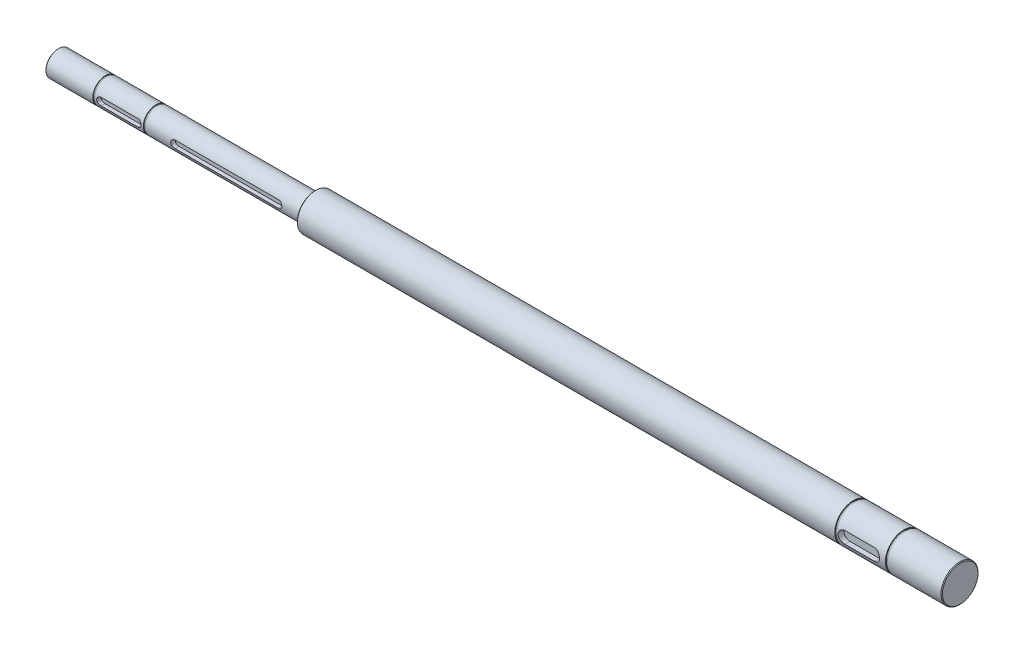
SolidWorks part; units mm, degrees
ref_plane "前视基准面" through (0, 0, 0) normal (0, 0, 1) x (1, 0, 0)
ref_plane "上视基准面" through (0, 0, 0) normal (0, 1, 0) x (1, 0, 0)
ref_plane "右视基准面" through (0, 0, 0) normal (1, 0, 0) x (0, 0, -1)
sketch "草图2" plane through (0, 0, 0) normal (1, 0, 0) x (0, 0, -1)
  circle A0 centre (0, 0) radius 12.5
  dimension "D1" = 25
extrude "凸台-拉伸1" add sketch "草图2" along normal mid plane 609
sketch "草图3" plane through (-304.5, 0, 0) normal (-1, 0, 0) x (0, 0, 1)
  circle A0 centre (0, 0) radius 8.5
  dimension "D1" = 17
extrude "切除-拉伸1" cut sketch "草图3" against normal blind 173.5 flip side to cut
ref_plane "基准面1" through (0, 0, 8.5) normal (0, 0, 1) x (1, 0, 0)
sketch "草图5" plane through (0, 0, 8.5) normal (0, 0, 1) x (1, 0, 0)
  line L0 (-267.5, 0) -> (-242.5, 0) construction
  line L1 (-267.5, 2.5) -> (-242.5, 2.5)
  line L2 (-267.5, -2.5) -> (-242.5, -2.5)
  line L3 (-217.5, 0) -> (-147.5, 0) construction
  line L4 (-217.5, 2.5) -> (-147.5, 2.5)
  line L5 (-217.5, -2.5) -> (-147.5, -2.5)
  line L7 (-304.5, 8.5) -> (-304.5, -8.5) construction
  arc A0 (-267.5, 2.5) -> (-267.5, -2.5) centre (-267.5, 0) ccw
  arc A1 (-242.5, -2.5) -> (-242.5, 2.5) centre (-242.5, 0) ccw
  arc A2 (-217.5, 2.5) -> (-217.5, -2.5) centre (-217.5, 0) ccw
  arc A3 (-147.5, -2.5) -> (-147.5, 2.5) centre (-147.5, 0) ccw
  point P3 (-255, 0)
  point P8 (-182.5, 0)
  dimension "D5" = 25
  dimension "D6" = 49.5
  dimension "D1" = 5
  dimension "D2" = 5
  dimension "D3" = 25
  dimension "D4" = 70
extrude "切除-拉伸2" cut sketch "草图5" against normal blind 3
ref_plane "基准面2" through (0, 0, 12.5) normal (0, 0, 1) x (1, 0, 0)
sketch "草图6" plane through (0, 0, 12.5) normal (0, 0, 1) x (1, 0, 0)
  line L0 (238.5, 0) -> (258.5, 0) construction
  line L1 (238.5, 4) -> (258.5, 4)
  line L2 (238.5, -4) -> (258.5, -4)
  line L3 (304.5, -12.5) -> (304.5, 12.5) construction
  arc A0 (238.5, 4) -> (238.5, -4) centre (238.5, 0) ccw
  arc A1 (258.5, -4) -> (258.5, 4) centre (258.5, 0) ccw
  point P3 (248.5, 0)
  dimension "D2" = 46
  dimension "D1" = 20
  dimension "D3" = 8
extrude "切除-拉伸3" cut sketch "草图6" against normal blind 4
chamfer "倒角1" distance 0.5 angle 45 2 edges at (304.5, 0, -12.5) (-131, 0, 12.5)
chamfer "倒角2" distance 0.3 angle 45 1 edges at (-304.5, 0, 8.5)
sketch "草图8" plane through (0, 0, 0) normal (0, 0, 1) x (1, 0, 0)
  line L0 (-130.5, -12.5) -> (304, -12.5) construction
  line L1 (267.7, -12.5) -> (266.5, -12.5)
  line L2 (267.7, -12.5) -> (267.7, -11.95)
  line L3 (267.7, -11.95) -> (266.5, -11.95)
  line L4 (266.5, -12.5) -> (266.5, -11.95)
  line L5 (304.5, -12) -> (304.5, 12) construction
  dimension "D1" = 1.2
  dimension "D2" = 0.55
  dimension "D3" = 36.8
revolve "切除-旋转2" cut sketch "草图8" angle 360 about axis through (304.5, 0, 0) along (-1, 0, 0)
pattern_linear "阵列(线性)2" count 2 spacing 34.2 along (-1, 0, 0) of "切除-旋转2"
sketch "草图9" plane through (0, 0, 0) normal (0, 0, 1) x (1, 0, 0)
  line L0 (-304.2, -8.5) -> (-131, -8.5) construction
  line L1 (-272.6, -8.5) -> (-271.5, -8.5)
  line L2 (-272.6, -8.5) -> (-272.6, -8.1)
  line L3 (-272.6, -8.1) -> (-271.5, -8.1)
  line L4 (-271.5, -8.5) -> (-271.5, -8.1)
  line L6 (-255, 2.5) -> (-255, -19.4569) construction
  line L7 (-242.5, 2.5) -> (-267.5, 2.5) construction
  dimension "D1" = 0.4
  dimension "D2" = 1.1
  dimension "D3" = 16.5
revolve "切除-旋转3" cut sketch "草图9" angle 360 about axis through (-131, 0, 0) along (-1, 0, 0)
pattern_linear "阵列(线性)3" count 2 spacing 34.1 along (1, 0, 0) of "切除-旋转3"
fillet "圆角1" radius 1.5 1 edges at (-131, 0, 8.5)
